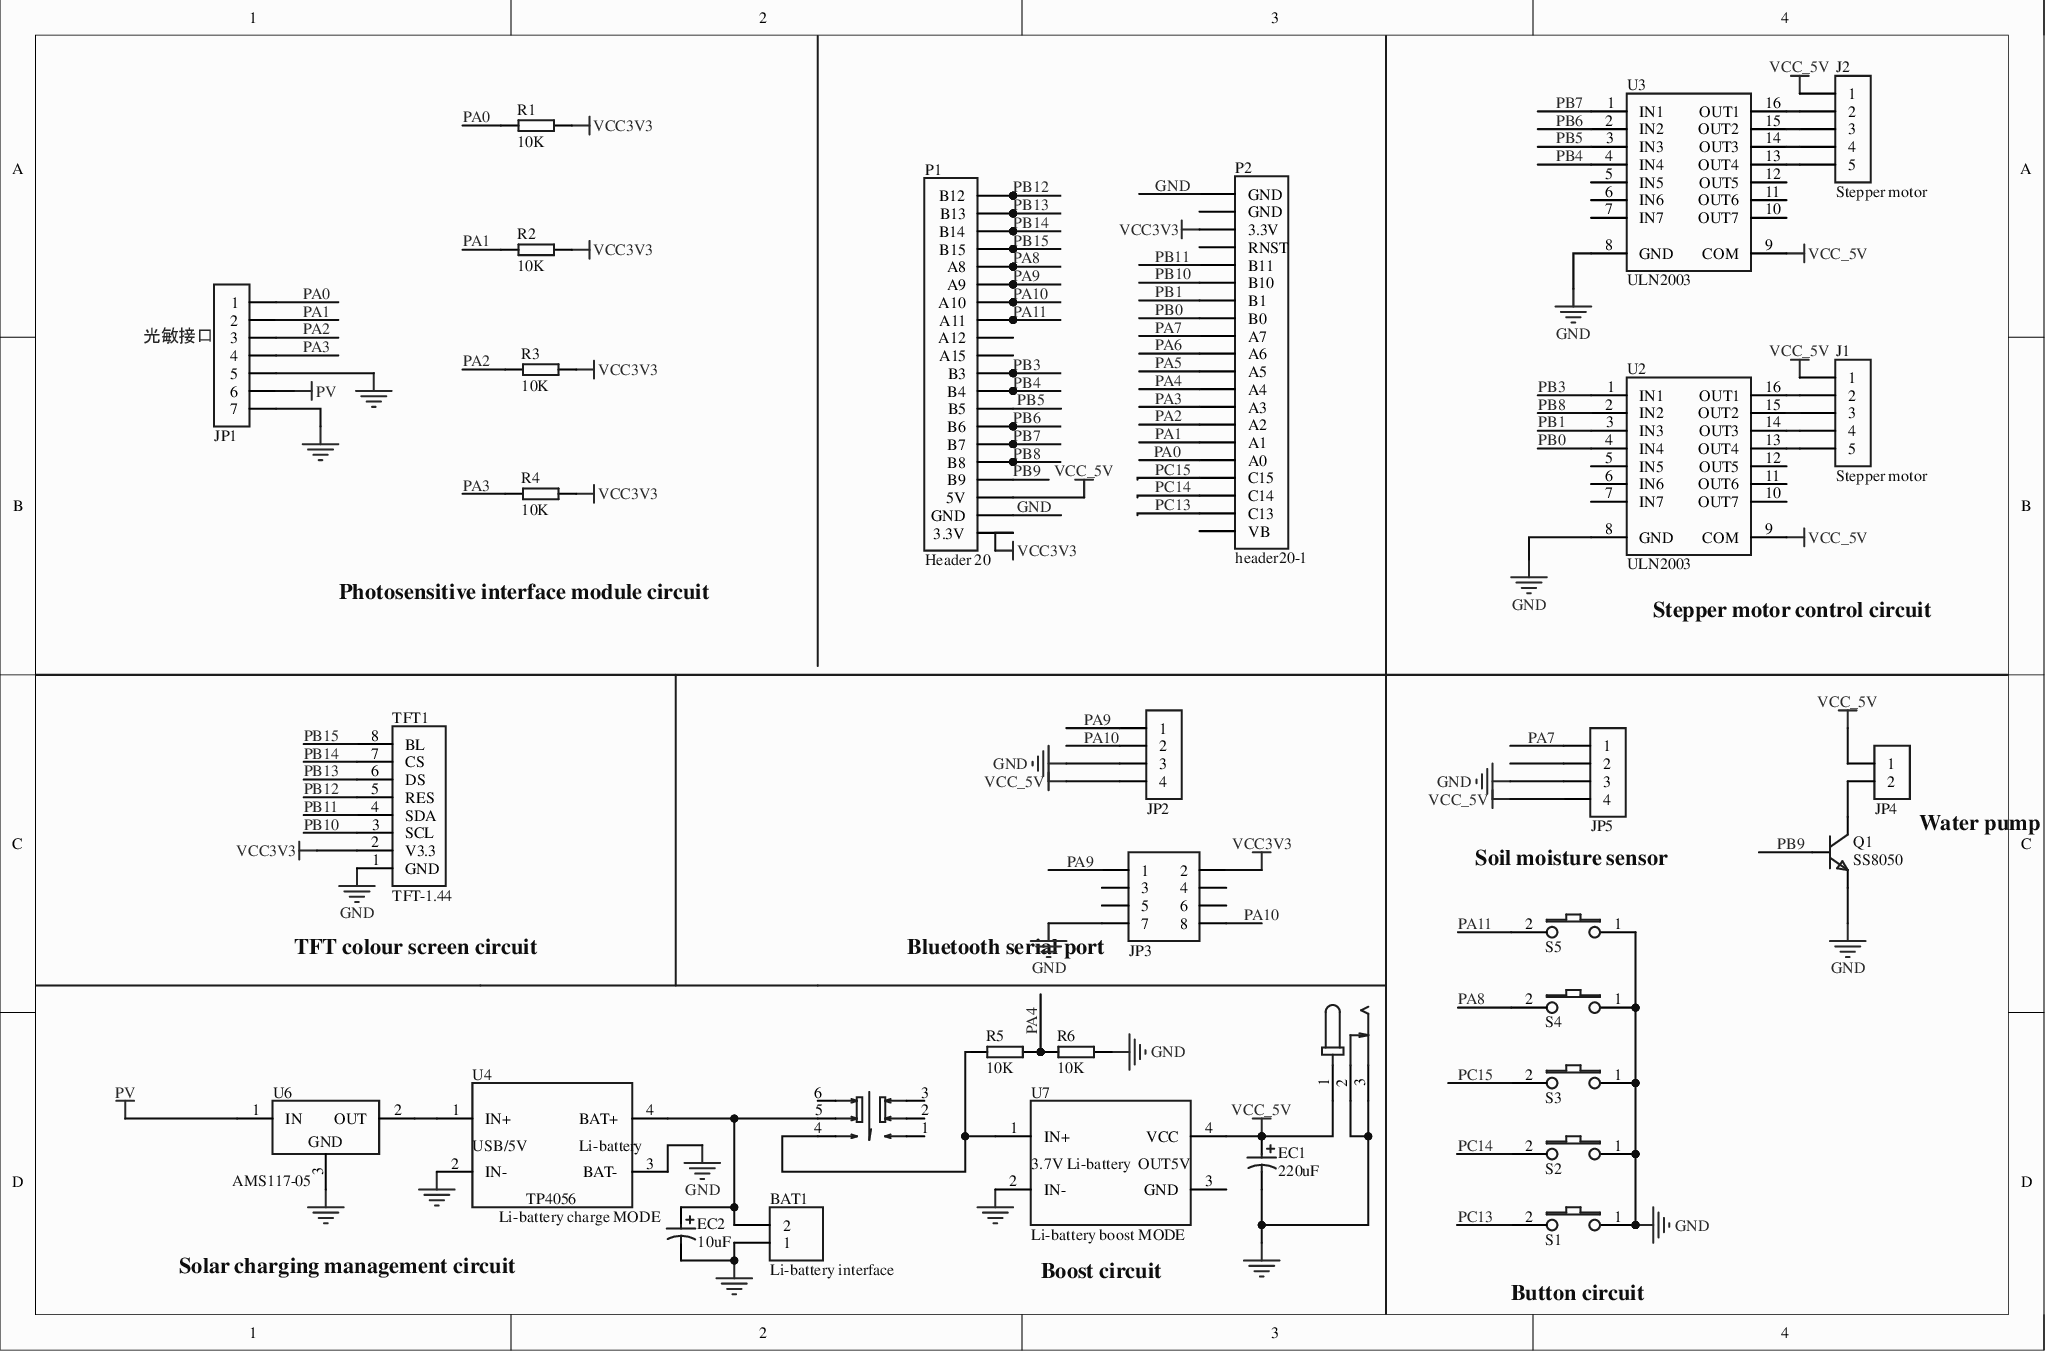
[diagram p0: MISC51567-3.schdoc]
# Altium project MISC51567-2.PrjPcb
1 sheet, 32 parts. Net scope: global (net labels, ports and power ports of the same name join across sheets).
Board file: MISC51567.pcbdoc

## Sheet MISC51567-3.schdoc
size 292 x 193 mm; SheetNumber: 1; SheetTotal: 1; Name: MISC51567

### Parts
BAT1  Li-battery interface  [CONN-TH_2P-P5.00_KF301-2P]
DC1  DC002-1.3  [DC-IN-TH_DC002-1.3]  (value not drawn)
EC1  220uF  [CAP-TH_BD10.0-P5.00-D0.6-FD]
EC2  10uF  [CAP-TH_BD5.0-P2.00-D0.8-FD-10UF50VC110GL]
J1  Stepper motor  [CONN-TH_5P-P2.54_C9900008095]
J2  Stepper motor  [CONN-TH_5P-P2.54_C9900008095]
JP1  HDR-1X7  [HDR-TH_7P-P2.54-V-F]  (value not drawn)
JP2  HDR-1X4  [HDR-TH_4P-P2.54-V-F]  (value not drawn)
JP3  Header 4X2  [HDR-TH_8P-P2.54-V-F-R2-C4-S2.54-1]  (value not drawn)
JP4  HDR-1X2  [HDR-TH_2P-P2.54-V-F]  (value not drawn)
JP5  HDR-1X4  [HDR-TH_4P-P2.54-V-F]  (value not drawn)
P1  Header 20  [HDR-TH_20P-P2.54-V-F]
P2  header20-1  [HDR-TH_20P-P2.54-V-F]
Q1  SS8050  [HDR-TH_3P-P2.54-V-F]
R1  10K  [Res_1/8W]
R2  10K  [Res_1/8W]
R3  10K  [Res_1/8W]
R4  10K  [Res_1/8W]
R5  10K  [Res_1/8W]
R6  10K  [Res_1/8W]
S1  BUTTOM  [SW-TH_4P-L6.0-W6.0-P4.50-LS6.5]  (value not drawn)
S2  BUTTOM  [SW-TH_4P-L6.0-W6.0-P4.50-LS6.5]  (value not drawn)
S3  BUTTOM  [SW-TH_4P-L6.0-W6.0-P4.50-LS6.5]  (value not drawn)
S4  BUTTOM  [SW-TH_4P-L6.0-W6.0-P4.50-LS6.5]  (value not drawn)
S5  BUTTOM  [SW-TH_4P-L6.0-W6.0-P4.50-LS6.5]  (value not drawn)
SW1  Self-lock button  [SW-TH_6P-L7.0-W7.0-P2.00]  (value not drawn)
TFT1  TFT-1.44  [CONN-TH_8P-P2.50_ZX-XH2.54-8PZZ-GW]
U2  ULN2003  [PDIP-16_L19.6-W6.5-P2.54-LS7.9-BL]
U3  ULN2003  [PDIP-16_L19.6-W6.5-P2.54-LS7.9-BL]
U4  Li-battery charge MODE  [JYMK]
U6  AMS117-05  [CONN-TH_3P-P2.54_8-102202-4]
U7  Li-battery boost MODE  [JYMK]

### Nets
GND: BAT1.1 DC1.2 DC1.3 EC1.2 EC2.2 JP1.5 JP1.7 JP2.3 JP3.7 JP5.3 P1.19(GND) P2.1(GND) Q1.1(E) R6.1 S1.1 S2.1 S3.1 S4.1 S5.1 TFT1.1(GND) U2.8(GND) U3.8(GND) U4.2(IN-) U4.3(BAT-) U6.3(GND) U7.2(IN-)
PV: JP1.6 U6.1(IN)
VCC3V3: JP3.2 P1.20(3.3V) P2.3(3.3V) R1.2 R2.2 R3.2 R4.2 TFT1.2(V3.3)
VCC_5V: DC1.1 EC1.1 J1.1 J2.1 JP2.4 JP4.1 JP5.4 P1.18(5V) U2.9(COM) U3.9(COM) U7.4(VCC)
PA0: JP1.1 P2.16(A0) R1.1
PA1: JP1.2 P2.15(A1) R2.1
PA2: JP1.3 P2.14(A2) R3.1
PA3: JP1.4 P2.13(A3) R4.1
PA4: P2.12(A4) R5.1 R6.2
PA5: P2.11(A5)
PA6: P2.10(A6)
PA7: JP5.1 P2.9(A7)
PA8: P1.5(A8) S4.2
PA9: JP2.1 JP3.1 P1.6(A9)
PA10: JP2.2 JP3.8 P1.7(A10)
PA11: P1.8(A11) S5.2
PB0: P2.8(B0) U2.4(IN4)
PB1: P2.7(B1) U2.3(IN3)
PB3: P1.11(B3) U2.1(IN1)
PB4: P1.12(B4) U3.4(IN4)
PB5: P1.13(B5) U3.3(IN3)
PB6: P1.14(B6) U3.2(IN2)
PB7: P1.15(B7) U3.1(IN1)
PB8: P1.16(B8) U2.2(IN2)
PB9: P1.17(B9) Q1.2(B)
PB10: P2.6(B10) TFT1.3(SCL)
PB11: P2.5(B11) TFT1.4(SDA)
PB12: P1.1(B12) TFT1.5(RES)
PB13: P1.2(B13) TFT1.6(DS)
PB14: P1.3(B14) TFT1.7(CS)
PB15: P1.4(B15) TFT1.8(BL)
PC13: P2.19(C13) S1.2
PC14: P2.18(C14) S2.2
PC15: P2.17(C15) S3.2
NetBAT1_2: BAT1.2 EC2.1 SW1.5 U4.4(BAT+)
NetJ1_2: J1.2 U2.16(OUT1)
NetJ1_3: J1.3 U2.15(OUT2)
NetJ1_4: J1.4 U2.14(OUT3)
NetJ1_5: J1.5 U2.13(OUT4)
NetJ2_2: J2.2 U3.16(OUT1)
NetJ2_3: J2.3 U3.15(OUT2)
NetJ2_4: J2.4 U3.14(OUT3)
NetJ2_5: J2.5 U3.13(OUT4)
NetJP4_2: JP4.2 Q1.3(C)
NetR5_2: R5.2 SW1.4 U7.1(IN+)
NetU4_1: U4.1(IN+) U6.2(OUT)

Not connected (* = marked no-connect by the designer): JP3 3 4 5 6; JP5 2; P1 9(A12) 10(A15); P2 2(GND) 4(RNST) 20(VB); SW1 1 2 3 6; U2 5(IN5) 6(IN6) 7(IN7) 10(OUT7) 11(OUT6) 12(OUT5); U3 5(IN5) 6(IN6) 7(IN7) 10(OUT7) 11(OUT6) 12(OUT5); U7 3(GND)*

### Notes on the sheet
- Photosensitive interface module circuit
- (near U2) Stepper motor control circuit
- Water pump
- Soil moisture sensor
- (near TFT1) TFT colour screen circuit
- (near JP3) Bluetooth serial port
- Solar charging management circuit
- (near U7) Boost circuit
- (near S1) Button circuit
- Labels drawn without touching a wire or pin: 光敏接口

### Library data of the parts
BAT1 = 锂电池接口: 2-pin terminal block; Origin Footprint: 5.08 two-pin terminal block; UniqueId: c8f831647f84318f; SymbolName: CON2; AddInBom: yes; Device: Li-battery interface; LatestRevisionDate: 17-Jul-2002; LatestRevisionNote: Re-released for DXP Platform.; DesignItemID: CON2; LibraryName: Reference; Publisher: Altium Limited
DC1 = DC002-1.3: Manufacturer: SHOU HAN(首韩); Add into BOM: yes; Connector Type: DC power jack; Inside Contact Diameter: 1.3mm; Outside Contact Diameter: 4.2mm; Current Rating (Max): 500mA; Voltage Rating (Max): 30V; UniqueId: 60d251d9786cec0c; ModelId: ccf1f99d79ab40ba9aeff26c21c7d5f1; Device: DC002-1.3; LCSC Part Name: DC电源插座 内径:1.3mm 外径:4.2mm; Supplier Part: C668593; Manufacturer Part: DC002-1.3; Supplier Footprint: 插件; JLCPCB Part Class: Extended Part; Datasheet: https://atta.szlcsc.com/upload/public/pdf/source/20200619/C668593_6B5785499F122503841AA69BD23A954B.pdf; Supplier: LCSC; Convert to PCB: yes; Mounting Style: Right-angle; Operating Temperature Range: -; DesignItemID: DC002-1.3; LibraryName: Schlib1; SymbolName: DC002-1.3; FootprintName: DC-IN-TH_DC002-1.3; ModelName: DC-IN-TH_DC002-1.3
EC1 = 220uF: Polarised capacitor; Origin Footprint: RB.15/.3; UniqueId: 1f6a804da79fa676; SymbolName: CAP_EC; AddInBom: yes; Device: 220uF; OriginFootprint 2: RB.15/.3; DesignItemID: CAP_EC; LibraryName: Reference
EC2 = 10uF: Polarised capacitor; Origin Footprint: RB.1/.2; UniqueId: b3a31b278d6dd2ce; SymbolName: CAP_EC; AddInBom: yes; Device: 10uF; DesignItemID: CAP_EC; LibraryName: Reference
J1 = 步进电机: Stepper motor interface; Origin Footprint: SIP5-2.54; UniqueId: 9f49826860c2c79d; AddInBom: yes; Device: Stepper motor; DesignItemID: 步进电机; LibraryName: Reference; SymbolName: Stepper motor
J2 = 步进电机: Stepper motor interface; Origin Footprint: SIP5-2.54; UniqueId: 42913bc3a3449998; AddInBom: yes; Device: Stepper motor; DesignItemID: 步进电机; LibraryName: Reference; SymbolName: Stepper motor
JP1 = HDR-1X7: 7P connector; 版权归属: Footprint library source: COMPANY_A; Origin Footprint: XH2.54-LI-7P; OriginFootprint 2: HDR2.54-LI-7P; OriginFootprint 3: HDR2.54-M-LI-7P; OriginFootprint 4: HDR2.54-WI-7P; OriginFootprint 5: HDR2.54-WS-7P; OriginFootprint 6: HDR2.54-Y-LI-7P; OriginFootprint 7: HDR2.54-M-WS-7P; OriginFootprint 8: KF2510-LI-7P; OriginFootprint 9: XH2.54-WS-7P; OriginFootprint 10: XH2.54-LS-7P; OriginFootprint 11: KF2EDGK-2.54-LI-7P; OriginFootprint 12: KF2EDGK-2.54-WI-7P; UniqueId: 3f7cd319db4ef0a6; SymbolName: Header 7; AddInBom: yes; Device: HDR-1X7; BOM名称: 7P connector; DesignItemID: Header 7; LibraryName: 5.3 - Connector, pitch 2.54 (100mil)
JP2 = HDR-1X4: 4P connector; 版权归属: Footprint library source: COMPANY_A; 学习资源: 最新版本发布; Origin Footprint: HDR2.54-LI-4P; UniqueId: e68233645d205bf0; SymbolName: Header 4; AddInBom: yes; Device: HDR-1X4; BOM名称: 4P connector; DesignItemID: Header 4; LibraryName: 5.4 - Connector, pitch 2.54 (100mil)
JP3 = Header 4X2: 4*2P connector; 版权归属: Footprint library source: COMPANY_A; Origin Footprint: HDR2.54-LI-2x4P; UniqueId: 79e19c811f88cad0; AddInBom: yes; Device: Header 4X2; BOM名称: 4*2P connector; DesignItemID: Header 4X2; LibraryName: 5.4 - Connector, pitch 2.54 (100mil); SymbolName: Header 4X2
JP4 = HDR-1X2: 2P connector; 版权归属: Footprint library source: COMPANY_A; Origin Footprint: HDR2.54-LI-2P; OriginFootprint 2: XH2.54-LI-2P; OriginFootprint 3: HDR2.54-M-LI-2P; OriginFootprint 4: HDR2.54-WI-2P; OriginFootprint 5: HDR2.54-WS-2P; OriginFootprint 6: HDR2.54-Y-LI-2P; OriginFootprint 7: HDR2.54-M-WS-2P; OriginFootprint 8: KF2510-LI-2P; OriginFootprint 9: XH2.54-WS-2P; OriginFootprint 10: XH2.54-LS-2P; OriginFootprint 11: KF2EDGK-2.54-LI-2P; OriginFootprint 12: KF2EDGK-2.54-WI-2P; UniqueId: 4916ee2a60fad895; SymbolName: Header 2; AddInBom: yes; Device: HDR-1X2; BOM名称: 2P connector; DesignItemID: Header 2; LibraryName: 5.3 - Connector, pitch 2.54 (100mil)
JP5 = HDR-1X4: 4P connector; 版权归属: Footprint library source: COMPANY_A; 学习资源: 最新版本发布; Origin Footprint: HDR2.54-LI-4P; UniqueId: 1fa703e6fb2f7410; SymbolName: Header 4; AddInBom: yes; Device: HDR-1X4; BOM名称: 4P connector; DesignItemID: Header 4; LibraryName: 5.4 - Connector, pitch 2.54 (100mil)
P1 = Header 20: Header, 20-Pin; Origin Footprint: HDR1X20; UniqueId: f88e3064cb77b82c; AddInBom: yes; Device: Header 20; LatestRevisionDate: 17-Jul-2002; LatestRevisionNote: Re-released for DXP Platform.; DesignItemID: Header 20; LibraryName: Schlib1; SymbolName: Header 20; Publisher: Altium Limited
P2 = header20-1: Origin Footprint: 20P; UniqueId: ddb6c992c6045fb8; AddInBom: yes; Device: header20-1; DesignItemID: header20-1; LibraryName: Schlib1; SymbolName: header20-1
Q1 = SS8050: High-frequency amplifier, NPN type; 版权归属: Footprint library source: COMPANY_A; 属性: 40V 1.5A 1W 100MHZ; Origin Footprint: TO92A; UniqueId: 047b734180970fea; SymbolName: 8050-DIP; AddInBom: yes; Device: SS8050; BOM名称: High-frequency amplifier, NPN type; DesignItemID: 8050-DIP; LibraryName: 0.4 - Transistor
R1 = 10K: Resistor; Origin Footprint: AXIAL0.3; UniqueId: 4e166b190d4de1c3; SymbolName: RES; AddInBom: yes; Device: 10K; DesignItemID: RES; LibraryName: Reference
R2 = 10K: Resistor; Origin Footprint: AXIAL0.3; UniqueId: 06442d24ab060343; SymbolName: RES; AddInBom: yes; Device: 10K; DesignItemID: RES; LibraryName: Reference
R3 = 10K: Resistor; Origin Footprint: AXIAL0.3; UniqueId: 6e26aea592918673; SymbolName: RES; AddInBom: yes; Device: 10K; DesignItemID: RES; LibraryName: Reference
R4 = 10K: Resistor; Origin Footprint: AXIAL0.3; UniqueId: 49359f7360e76581; SymbolName: RES; AddInBom: yes; Device: 10K; DesignItemID: RES; LibraryName: Reference
R5 = 10K: Resistor; Origin Footprint: AXIAL0.3; UniqueId: 96bd3269827a783e; SymbolName: RES; AddInBom: yes; Device: 10K; DesignItemID: RES; LibraryName: Reference
R6 = 10K: Resistor; Origin Footprint: AXIAL0.3; UniqueId: c9a24d22ca7022dc; SymbolName: RES; AddInBom: yes; Device: 10K; DesignItemID: RES; LibraryName: Reference
S1 = BUTTOM: Button; Origin Footprint: BUTTOM_6x6DIP; UniqueId: da892dff24010eb4; AddInBom: yes; Device: BUTTOM; DesignItemID: BUTTOM; LibraryName: Reference; SymbolName: BUTTOM
S2 = BUTTOM: Button; Origin Footprint: BUTTOM_6x6DIP; UniqueId: b3b756e6393b620b; AddInBom: yes; Device: BUTTOM; DesignItemID: BUTTOM; LibraryName: Reference; SymbolName: BUTTOM
S3 = BUTTOM: Button; Origin Footprint: BUTTOM_6x6DIP; UniqueId: 7b79a888bb89fb64; AddInBom: yes; Device: BUTTOM; DesignItemID: BUTTOM; LibraryName: Reference; SymbolName: BUTTOM
S4 = BUTTOM: Button; Origin Footprint: BUTTOM_6x6DIP; UniqueId: 5bcf7e05ad3bc526; AddInBom: yes; Device: BUTTOM; DesignItemID: BUTTOM; LibraryName: Reference; SymbolName: BUTTOM
S5 = BUTTOM: Button; Origin Footprint: BUTTOM_6x6DIP; UniqueId: 3819b3f665fa52ad; AddInBom: yes; Device: BUTTOM; DesignItemID: BUTTOM; LibraryName: Reference; SymbolName: BUTTOM
SW1 = 自锁按键: Manufacturer: XKB Connectivity(中国星坤); Manufacturer Part: XKB7070-Z; Add into BOM: yes; Actuator Style: Rectangular button; Contact Current: 100mA; Voltage Rating (AC): 250V; Voltage Rating (DC): 30V; Insulation Resistance: 100MΩ; Actuator/Cap Color: Blue; With Lamp: Without; Pin Style: PC pin; Operating Force: 160gf; Mechanical Life: 10万 cycles; UniqueId: 1070c7afd779bef2; ModelId: 65f5674ceb7247f197b01bc7adea0d8f; Device: Self-lock button; LCSC Part Name: 按键开关   7*7插件自锁 蓝白黑; Supplier Part: C318863; Supplier Footprint: 插件; JLCPCB Part Class: Extended Part; Datasheet: https://atta.szlcsc.com/upload/public/pdf/source/20211015/75A682A27A424BDE8D93C2CFA14C38FE.pdf; Supplier: LCSC; Convert to PCB: yes; Self Lock / No Lock: Self-lock; IP Rating: -; Mounting Style: Through-hole; Operating Temperature: -15℃~+55℃; DesignItemID: XKB7070-Z; LibraryName: Schlib1; SymbolName: XKB7070-Z; FootprintName: SW-TH_6P-L7.0-W7.0-P2.00; ModelName: SW-TH_6P-L7.0-W7.0-P2.00
TFT1 = TFT-1.44: Origin Footprint: 8Pin header replaces TFT colour screen; OriginFootprint 2: HDR-TH_8P-P2.54-V-M; UniqueId: 452982523a522371; AddInBom: yes; Device: TFT-1.44; OriginFootprint 3: TFT-1.44; DesignItemID: TFT-1.44; LibraryName: Reference; Description: TFT-1.44; SymbolName: TFT-1.44
U2 = ULN2003: ULN2003 chip; Origin Footprint: DIP16; UniqueId: d74c11912b695046; SymbolName: ULN2003A; AddInBom: yes; Device: ULN2003; DesignItemID: ULN2003A; LibraryName: Reference
U3 = ULN2003: ULN2003 chip; Origin Footprint: DIP16; UniqueId: eac3f191c372887e; SymbolName: ULN2003A; AddInBom: yes; Device: ULN2003; DesignItemID: ULN2003A; LibraryName: Reference
U4 = 锂电充电MODE: Li-battery charge control module; Origin Footprint: TP4056_MODE; UniqueId: e5d1bee62801ccc5; AddInBom: yes; Device: Li-battery charge MODE; DesignItemID: 锂电池充电MODE; LibraryName: Reference; SymbolName: Li-battery charge MODE
U6 = AMS117-05: 7805 regulator chip; Origin Footprint: HDR2.54-LI-3P; UniqueId: cb0a5e759a2bc85d; SymbolName: LM78M05; AddInBom: yes; Device: AMS117-05; DesignItemID: LM78M05; LibraryName: Reference
U7 = 锂电池升压MODE: Li-battery boost module; Origin Footprint: USB_UPVOLT; UniqueId: 917392894f3a2a5c; AddInBom: yes; Device: Li-battery boost MODE; DesignItemID: 锂电池升压MODE; LibraryName: Reference; SymbolName: Li-battery boost MODE